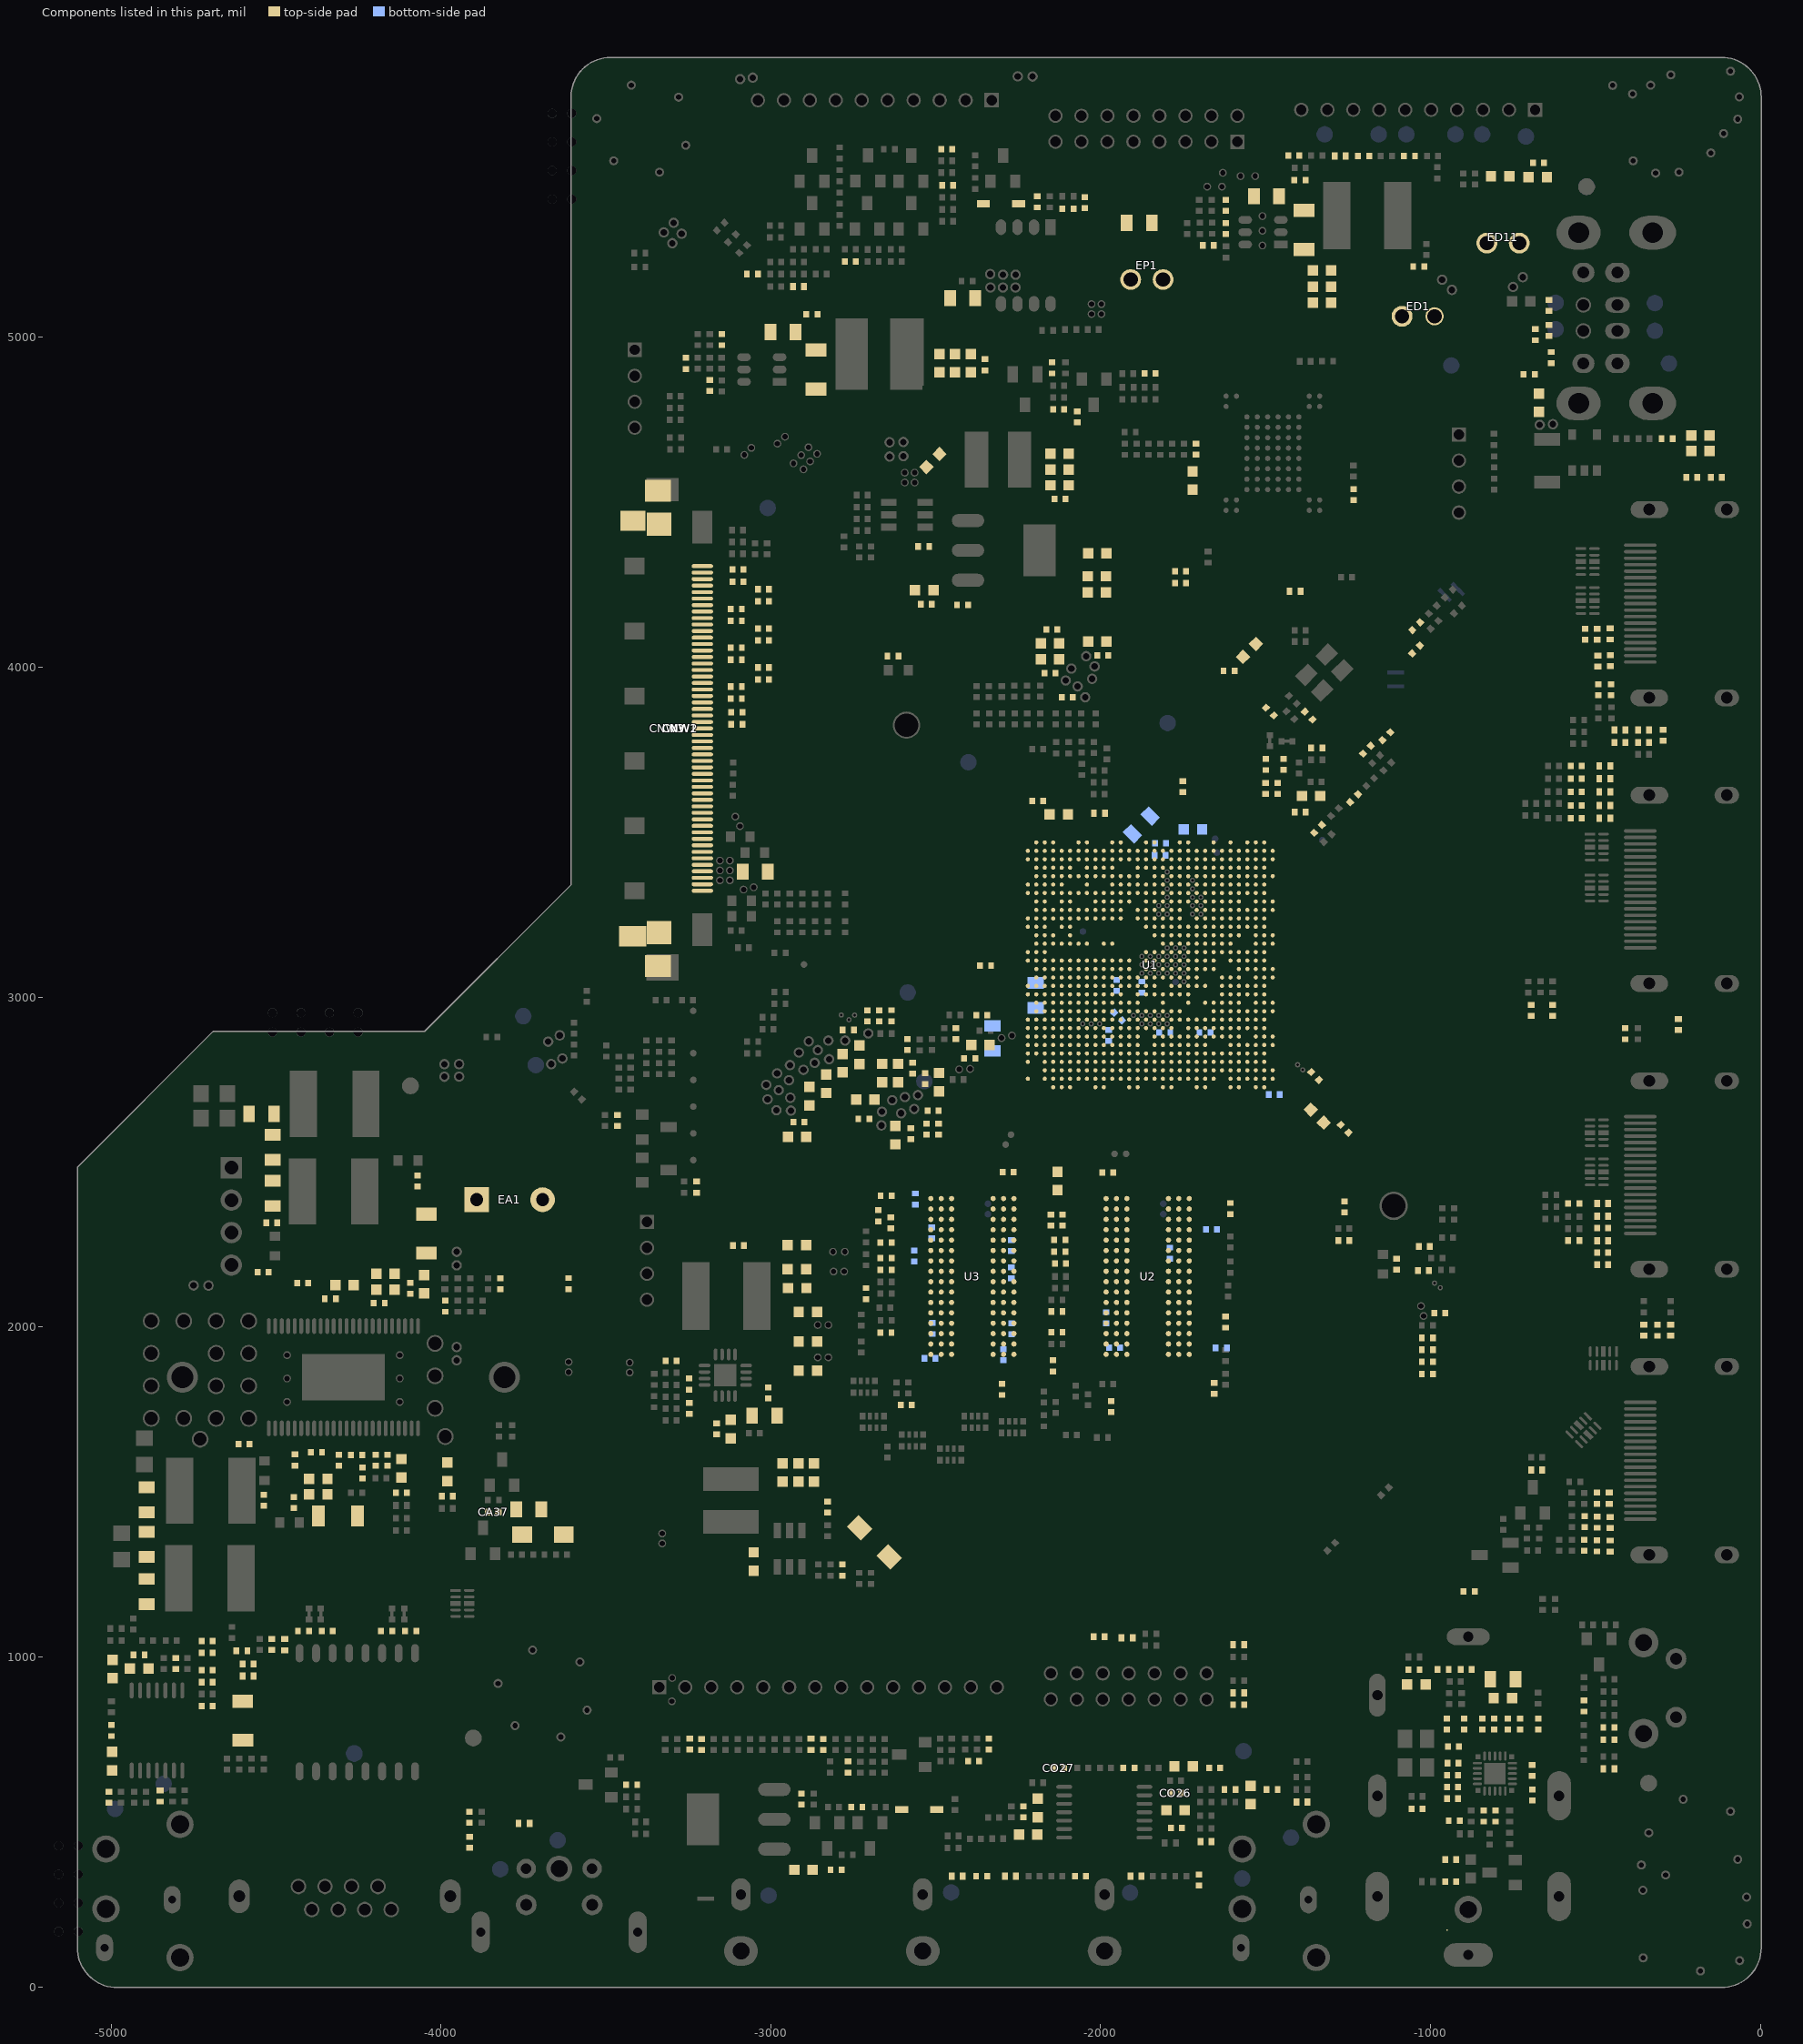
[diagram p0: the components of this part, seen from the top]
# Altium PCB MISC86290.PcbDoc (part 5 of 31)
Units mil, origin at the board's own origin, x right, y up, seen from the top; angles counter-clockwise.
Board outline 5104.71 x 5851.49 mil, 2 copper layers (TopLayer, BottomLayer), stack 61.855 mil thick; 1026 components, 667 nets, 4280 pads, 2294 vias.

## Footprints (in the part's own frame and the unit in brackets; to place one, negate y for a bottom-side part, rotate by r counter-clockwise, add the part's x,y. Pads: shape width x height; smd on the part's side, far side on the other; paste and mask are expansions set on the pad) (continued)
BGA96/0.8-1 [mm] "SKhynix；4GB DDR3 SDRAM　 9.4*13／NANYA　SDRAM B-Die　10*13兼容"
  round 0.4 smd: A1(-3.2,6) A2(-2.4,6) A3(-1.6,6) A7(1.6,6) A8(2.4,6) A9(3.2,6) B1(-3.2,5.2) B2(-2.4,5.2) B3(-1.6,5.2) B7(1.6,5.2) B8(2.4,5.2) B9(3.2,5.2) C1(-3.2,4.4) C2(-2.4,4.4) C3(-1.6,4.4) C7(1.6,4.4) C8(2.4,4.4) C9(3.2,4.4) D1(-3.2,3.6) D2(-2.4,3.6) D3(-1.6,3.6) D7(1.6,3.6) D8(2.4,3.6) D9(3.2,3.6) E1(-3.2,2.8) E2(-2.4,2.8) E3(-1.6,2.8) E7(1.6,2.8) E8(2.4,2.8) E9(3.2,2.8) F1(-3.2,2) F2(-2.4,2) F3(-1.6,2) F7(1.6,2) F8(2.4,2) F9(3.2,2) G1(-3.2,1.2) G2(-2.4,1.2) G3(-1.6,1.2) G7(1.6,1.2) G8(2.4,1.2) G9(3.2,1.2) H1(-3.2,0.4) H2(-2.4,0.4) H3(-1.6,0.4) H7(1.6,0.4) H8(2.4,0.4) H9(3.2,0.4) J1(-3.2,-0.4) J2(-2.4,-0.4) J3(-1.6,-0.4) J7(1.6,-0.4) J8(2.4,-0.4) J9(3.2,-0.4) K1(-3.2,-1.2) K2(-2.4,-1.2) K3(-1.6,-1.2) K7(1.6,-1.2) K8(2.4,-1.2) K9(3.2,-1.2) L1(-3.2,-2) L2(-2.4,-2) L3(-1.6,-2) L7(1.6,-2) L8(2.4,-2) L9(3.2,-2) M1(-3.2,-2.8) M2(-2.4,-2.8) M3(-1.6,-2.8) M7(1.6,-2.8) M8(2.4,-2.8) M9(3.2,-2.8) N1(-3.2,-3.6) N2(-2.4,-3.6) N3(-1.6,-3.6) N7(1.6,-3.6) N8(2.4,-3.6) N9(3.2,-3.6) P1(-3.2,-4.4) P2(-2.4,-4.4) P3(-1.6,-4.4) P7(1.6,-4.4) P8(2.4,-4.4) P9(3.2,-4.4) R1(-3.2,-5.2) R2(-2.4,-5.2) R3(-1.6,-5.2) R7(1.6,-5.2) R8(2.4,-5.2) R9(3.2,-5.2) T1(-3.2,-6) T2(-2.4,-6) T3(-1.6,-6) T7(1.6,-6) T8(2.4,-6) T9(3.2,-6)
  silkscreen extent -5.59,-6.7 5.05,7.49, body extent -5.05,-6.55 5.05,6.55, height 1.2
BGA758/0.65 [mm] "Mstar,MSDURN1801-Z1,0822_2018"
  round 0.32 smd mask+0.051: A2(-8.775,9.425) A3(-8.125,9.425) A5(-6.825,9.425) A6(-6.175,9.425) A9(-4.225,9.425) A10(-3.575,9.425) A13(-1.625,9.425) A14(-0.975,9.425) A17(0.975,9.425) A18(1.625,9.425) A21(3.575,9.425) A22(4.225,9.425) A25(6.175,9.425) A26(6.825,9.425) A27(7.475,9.425) AA2(-8.775,-3.575) AA3(-8.125,-3.575) AA4(-7.475,-3.575) AA5(-6.825,-3.575) AA6(-6.175,-3.575) AA7(-5.525,-3.575) AA8(-4.875,-3.575) AA9(-4.225,-3.575) AA10(-3.575,-3.575) AA12(-2.275,-3.575) AA13(-1.625,-3.575) AA14(-0.975,-3.575) AA15(-0.325,-3.575) AA16(0.325,-3.575) AA17(0.975,-3.575) AA19(2.275,-3.575) AA20(2.925,-3.575) AA21(3.575,-3.575) AA22(4.225,-3.575) AA23(4.875,-3.575) AA24(5.525,-3.575) AA25(6.175,-3.575) AA26(6.825,-3.575) AA27(7.475,-3.575) AA28(8.125,-3.575) AA29(8.775,-3.575) AA30(9.425,-3.575) AB1(-9.425,-4.225) AB2(-8.775,-4.225) AB3(-8.125,-4.225) AB4(-7.475,-4.225) AB5(-6.825,-4.225) AB6(-6.175,-4.225) AB7(-5.525,-4.225) AB8(-4.875,-4.225) AB9(-4.225,-4.225) AB10(-3.575,-4.225) AB12(-2.275,-4.225) AB13(-1.625,-4.225) AB14(-0.975,-4.225) AB15(-0.325,-4.225) AB16(0.325,-4.225) AB17(0.975,-4.225) AB19(2.275,-4.225) AB20(2.925,-4.225) AB21(3.575,-4.225) AB22(4.225,-4.225) AB23(4.875,-4.225) AB24(5.525,-4.225) AB25(6.175,-4.225) AB26(6.825,-4.225) AB27(7.475,-4.225) AB28(8.125,-4.225) AB29(8.775,-4.225) AC1(-9.425,-4.875) AC2(-8.775,-4.875) AC3(-8.125,-4.875) AC5(-6.825,-4.875) AC6(-6.175,-4.875) AC7(-5.525,-4.875) AC8(-4.875,-4.875) AC9(-4.225,-4.875) AC10(-3.575,-4.875) AC11(-2.925,-4.875) AC12(-2.275,-4.875) AC13(-1.625,-4.875) AC14(-0.975,-4.875) AC15(-0.325,-4.875) AC16(0.325,-4.875) AC18(1.625,-4.875) AC19(2.275,-4.875) AC20(2.925,-4.875) AC21(3.575,-4.875) AC22(4.225,-4.875) AC25(6.175,-4.875) AC26(6.825,-4.875) AC28(8.125,-4.875) AC29(8.775,-4.875) AD2(-8.775,-5.525) AD3(-8.125,-5.525) AD4(-7.475,-5.525) AD5(-6.825,-5.525) AD6(-6.175,-5.525) AD7(-5.525,-5.525) AD8(-4.875,-5.525) AD9(-4.225,-5.525) AD10(-3.575,-5.525) AD11(-2.925,-5.525) AD12(-2.275,-5.525) AD13(-1.625,-5.525) AD14(-0.975,-5.525) AD15(-0.325,-5.525) AD16(0.325,-5.525) AD17(0.975,-5.525) AD18(1.625,-5.525) AD19(2.275,-5.525) AD20(2.925,-5.525) AD21(3.575,-5.525) AD22(4.225,-5.525) AD23(4.875,-5.525) AD24(5.525,-5.525) AD25(6.175,-5.525) AD26(6.825,-5.525) AD27(7.475,-5.525) AD28(8.125,-5.525) AD29(8.775,-5.525) AD30(9.425,-5.525) AE2(-8.775,-6.175) AE3(-8.125,-6.175) AE4(-7.475,-6.175) AE5(-6.825,-6.175) AE6(-6.175,-6.175) AE7(-5.525,-6.175) AE8(-4.875,-6.175) AE9(-4.225,-6.175) AE10(-3.575,-6.175) AE11(-2.925,-6.175) AE12(-2.275,-6.175) AE13(-1.625,-6.175) AE14(-0.975,-6.175) AE15(-0.325,-6.175) AE16(0.325,-6.175) AE17(0.975,-6.175) AE18(1.625,-6.175) AE19(2.275,-6.175) AE20(2.925,-6.175) AE23(4.875,-6.175) AE26(6.825,-6.175) AE27(7.475,-6.175) AE28(8.125,-6.175) AE29(8.775,-6.175) AE30(9.425,-6.175) AF1(-9.425,-6.825) AF2(-8.775,-6.825) AF3(-8.125,-6.825) AF4(-7.475,-6.825) AF5(-6.825,-6.825) AF6(-6.175,-6.825) AF7(-5.525,-6.825) AF8(-4.875,-6.825) AF9(-4.225,-6.825) AF10(-3.575,-6.825) AF11(-2.925,-6.825) AF12(-2.275,-6.825) AF13(-1.625,-6.825) AF14(-0.975,-6.825) AF15(-0.325,-6.825) AF17(0.975,-6.825) AF18(1.625,-6.825) AF19(2.275,-6.825) AF20(2.925,-6.825) AF21(3.575,-6.825) AF22(4.225,-6.825) AF23(4.875,-6.825) AF24(5.525,-6.825) AF25(6.175,-6.825) AF26(6.825,-6.825) AF27(7.475,-6.825) AF28(8.125,-6.825) AF29(8.775,-6.825) AG2(-8.775,-7.475) AG3(-8.125,-7.475) AG4(-7.475,-7.475) AG5(-6.825,-7.475) AG6(-6.175,-7.475) AG7(-5.525,-7.475) AG8(-4.875,-7.475) AG9(-4.225,-7.475) AG10(-3.575,-7.475) AG11(-2.925,-7.475) AG12(-2.275,-7.475) AG13(-1.625,-7.475) AG14(-0.975,-7.475) AG15(-0.325,-7.475) AG16(0.325,-7.475) AG17(0.975,-7.475) AG20(2.925,-7.475) AG21(3.575,-7.475) AG22(4.225,-7.475) AG23(4.875,-7.475) AG25(6.175,-7.475) AG26(6.825,-7.475) AG27(7.475,-7.475) AG28(8.125,-7.475) AG29(8.775,-7.475) AH1(-9.425,-8.125) AH2(-8.775,-8.125) AH3(-8.125,-8.125) AH4(-7.475,-8.125) AH5(-6.825,-8.125) AH6(-6.175,-8.125) AH7(-5.525,-8.125) AH8(-4.875,-8.125) AH9(-4.225,-8.125) AH10(-3.575,-8.125) AH11(-2.925,-8.125) AH12(-2.275,-8.125) AH13(-1.625,-8.125) AH14(-0.975,-8.125) AH15(-0.325,-8.125) AH16(0.325,-8.125) AH17(0.975,-8.125) AH18(1.625,-8.125) AH19(2.275,-8.125) AH20(2.925,-8.125) AH21(3.575,-8.125) AH22(4.225,-8.125) AH23(4.875,-8.125) AH24(5.525,-8.125) AH25(6.175,-8.125) AH26(6.825,-8.125) AH27(7.475,-8.125) AH28(8.125,-8.125) AH29(8.775,-8.125) AH30(9.425,-8.125) AJ1(-9.425,-8.775) AJ2(-8.775,-8.775) AJ3(-8.125,-8.775) AJ4(-7.475,-8.775) AJ5(-6.825,-8.775) AJ6(-6.175,-8.775) AJ7(-5.525,-8.775) AJ8(-4.875,-8.775) AJ9(-4.225,-8.775) AJ10(-3.575,-8.775) AJ11(-2.925,-8.775) AJ12(-2.275,-8.775) AJ13(-1.625,-8.775) AJ14(-0.975,-8.775) AJ15(-0.325,-8.775) AJ16(0.325,-8.775) AJ17(0.975,-8.775) AJ18(1.625,-8.775) AJ19(2.275,-8.775) AJ20(2.925,-8.775) AJ21(3.575,-8.775) AJ22(4.225,-8.775) AJ23(4.875,-8.775) AJ24(5.525,-8.775) AJ25(6.175,-8.775) AJ26(6.825,-8.775) AJ27(7.475,-8.775) AJ28(8.125,-8.775) AJ29(8.775,-8.775) AJ30(9.425,-8.775) AK2(-8.775,-9.425) AK3(-8.125,-9.425) AK4(-7.475,-9.425) AK6(-6.175,-9.425) AK8(-4.875,-9.425) AK11(-2.925,-9.425) AK12(-2.275,-9.425) AK15(-0.325,-9.425) AK16(0.325,-9.425) AK19(2.275,-9.425) AK20(2.925,-9.425) AK23(4.875,-9.425) AK24(5.525,-9.425) AK27(7.475,-9.425) AK28(8.125,-9.425) AK29(8.775,-9.425) B1(-9.425,8.775) B2(-8.775,8.775) B3(-8.125,8.775) B4(-7.475,8.775) B5(-6.825,8.775) B6(-6.175,8.775) B8(-4.875,8.775) B9(-4.225,8.775) B10(-3.575,8.775) B11(-2.925,8.775) B12(-2.275,8.775) B13(-1.625,8.775) B14(-0.975,8.775) B15(-0.325,8.775) B16(0.325,8.775) B17(0.975,8.775) B18(1.625,8.775) B19(2.275,8.775) B20(2.925,8.775) B21(3.575,8.775) B22(4.225,8.775) B23(4.875,8.775) B24(5.525,8.775) B25(6.175,8.775) B26(6.825,8.775) B27(7.475,8.775) B28(8.125,8.775) B30(9.425,8.775) C1(-9.425,8.125) C2(-8.775,8.125) C3(-8.125,8.125) C4(-7.475,8.125) C5(-6.825,8.125) C6(-6.175,8.125) C7(-5.525,8.125) C8(-4.875,8.125) C9(-4.225,8.125) C10(-3.575,8.125) C11(-2.925,8.125) C12(-2.275,8.125) C13(-1.625,8.125) C14(-0.975,8.125) C15(-0.325,8.125) C16(0.325,8.125) C17(0.975,8.125) C18(1.625,8.125) C19(2.275,8.125) C20(2.925,8.125) C21(3.575,8.125) C22(4.225,8.125) C23(4.875,8.125) C24(5.525,8.125) C25(6.175,8.125) C26(6.825,8.125) C27(7.475,8.125) C28(8.125,8.125) D2(-8.775,7.475) D3(-8.125,7.475) D4(-7.475,7.475) D5(-6.825,7.475) D6(-6.175,7.475) D7(-5.525,7.475) D8(-4.875,7.475) D9(-4.225,7.475) D10(-3.575,7.475) D11(-2.925,7.475) D12(-2.275,7.475) D13(-1.625,7.475) D14(-0.975,7.475) D15(-0.325,7.475) D16(0.325,7.475) D17(0.975,7.475) D18(1.625,7.475) D19(2.275,7.475) D20(2.925,7.475) D21(3.575,7.475) D22(4.225,7.475) D23(4.875,7.475) D24(5.525,7.475) D25(6.175,7.475) D26(6.825,7.475) D27(7.475,7.475) D28(8.125,7.475) D30(9.425,7.475) E2(-8.775,6.825) E3(-8.125,6.825) E4(-7.475,6.825) E5(-6.825,6.825) E6(-6.175,6.825) E7(-5.525,6.825) E8(-4.875,6.825) E9(-4.225,6.825) E10(-3.575,6.825) E11(-2.925,6.825) E12(-2.275,6.825) E13(-1.625,6.825) E14(-0.975,6.825) E15(-0.325,6.825) E16(0.325,6.825) E17(0.975,6.825) E18(1.625,6.825) E19(2.275,6.825) E20(2.925,6.825) E21(3.575,6.825) E22(4.225,6.825) E23(4.875,6.825) E24(5.525,6.825) E25(6.175,6.825) E26(6.825,6.825) E27(7.475,6.825) E28(8.125,6.825) E29(8.775,6.825) E30(9.425,6.825) F1(-9.425,6.175) F2(-8.775,6.175) F3(-8.125,6.175) F4(-7.475,6.175) F5(-6.825,6.175) F6(-6.175,6.175) F9(-4.225,6.175) F10(-3.575,6.175) F11(-2.925,6.175) F12(-2.275,6.175) F13(-1.625,6.175) F14(-0.975,6.175) F15(-0.325,6.175) F17(0.975,6.175) F18(1.625,6.175) F19(2.275,6.175) F20(2.925,6.175) F21(3.575,6.175) F22(4.225,6.175) F23(4.875,6.175) F24(5.525,6.175) F25(6.175,6.175) F26(6.825,6.175) F27(7.475,6.175) F28(8.125,6.175) F29(8.775,6.175) F30(9.425,6.175) G1(-9.425,5.525) G2(-8.775,5.525) G3(-8.125,5.525) G5(-6.825,5.525) G6(-6.175,5.525) G7(-5.525,5.525) G8(-4.875,5.525) G9(-4.225,5.525) G10(-3.575,5.525) G11(-2.925,5.525) G12(-2.275,5.525) G13(-1.625,5.525) G14(-0.975,5.525) G15(-0.325,5.525) G17(0.975,5.525) G18(1.625,5.525) G19(2.275,5.525) G20(2.925,5.525) G21(3.575,5.525) G22(4.225,5.525) G23(4.875,5.525) G24(5.525,5.525) G25(6.175,5.525) G26(6.825,5.525) G27(7.475,5.525) G28(8.125,5.525) G29(8.775,5.525) G30(9.425,5.525) H2(-8.775,4.875) H3(-8.125,4.875) H4(-7.475,4.875) H5(-6.825,4.875) H6(-6.175,4.875) H7(-5.525,4.875) H8(-4.875,4.875) H9(-4.225,4.875) H10(-3.575,4.875) H11(-2.925,4.875) H13(-1.625,4.875) H14(-0.975,4.875) H15(-0.325,4.875) H16(0.325,4.875) H17(0.975,4.875) H18(1.625,4.875) H19(2.275,4.875) H20(2.925,4.875) H21(3.575,4.875) H22(4.225,4.875) H23(4.875,4.875) H24(5.525,4.875) H25(6.175,4.875) H26(6.825,4.875) H27(7.475,4.875) H28(8.125,4.875) H29(8.775,4.875) H30(9.425,4.875) J2(-8.775,4.225) J3(-8.125,4.225) J4(-7.475,4.225) J5(-6.825,4.225) J6(-6.175,4.225) J7(-5.525,4.225) J8(-4.875,4.225) J9(-4.225,4.225) J10(-3.575,4.225) J11(-2.925,4.225) J12(-2.275,4.225) J13(-1.625,4.225) J14(-0.975,4.225) J15(-0.325,4.225) J16(0.325,4.225) J17(0.975,4.225) J18(1.625,4.225) J19(2.275,4.225) J20(2.925,4.225) J21(3.575,4.225) J22(4.225,4.225) J23(4.875,4.225) J24(5.525,4.225) J25(6.175,4.225) J26(6.825,4.225) J27(7.475,4.225) J28(8.125,4.225) J29(8.775,4.225) J30(9.425,4.225) K1(-9.425,3.575) K2(-8.775,3.575) K3(-8.125,3.575) K4(-7.475,3.575) K5(-6.825,3.575) K6(-6.175,3.575) K7(-5.525,3.575) K8(-4.875,3.575) K12(-2.275,3.575) K13(-1.625,3.575) K14(-0.975,3.575) K15(-0.325,3.575) K16(0.325,3.575) K17(0.975,3.575) K18(1.625,3.575) K19(2.275,3.575) K20(2.925,3.575) K21(3.575,3.575) K22(4.225,3.575) K23(4.875,3.575) K24(5.525,3.575) K25(6.175,3.575) K26(6.825,3.575) K27(7.475,3.575) K28(8.125,3.575) K29(8.775,3.575) L1(-9.425,2.925) L2(-8.775,2.925) L3(-8.125,2.925) L5(-6.825,2.925) L6(-6.175,2.925) L7(-5.525,2.925) L8(-4.875,2.925) L9(-4.225,2.925) L11(-2.925,2.925) L14(-0.975,2.925) L17(0.975,2.925) L18(1.625,2.925) L19(2.275,2.925) L20(2.925,2.925) L21(3.575,2.925) L22(4.225,2.925) L23(4.875,2.925) L24(5.525,2.925) L25(6.175,2.925) L26(6.825,2.925) L27(7.475,2.925) L28(8.125,2.925) L29(8.775,2.925) M2(-8.775,2.275) M3(-8.125,2.275) M4(-7.475,2.275) M5(-6.825,2.275) M6(-6.175,2.275) M7(-5.525,2.275) M11(-2.925,2.275) M12(-2.275,2.275) M13(-1.625,2.275) M14(-0.975,2.275) M15(-0.325,2.275) M16(0.325,2.275) M17(0.975,2.275) M19(2.275,2.275) M20(2.925,2.275) M21(3.575,2.275) M22(4.225,2.275) M23(4.875,2.275) M24(5.525,2.275) M25(6.175,2.275) M26(6.825,2.275) M27(7.475,2.275) M28(8.125,2.275) M29(8.775,2.275) M30(9.425,2.275) N2(-8.775,1.625) N3(-8.125,1.625) N4(-7.475,1.625) N5(-6.825,1.625) N6(-6.175,1.625) N7(-5.525,1.625) N9(-4.225,1.625) N10(-3.575,1.625) N11(-2.925,1.625) N12(-2.275,1.625) N13(-1.625,1.625) N15(-0.325,1.625) N16(0.325,1.625) N17(0.975,1.625) N18(1.625,1.625) N19(2.275,1.625) N20(2.925,1.625) N21(3.575,1.625) N22(4.225,1.625) N23(4.875,1.625) N24(5.525,1.625) N25(6.175,1.625) N26(6.825,1.625) N27(7.475,1.625) N28(8.125,1.625) N29(8.775,1.625) N30(9.425,1.625) P1(-9.425,0.975) P2(-8.775,0.975) P3(-8.125,0.975) P5(-6.825,0.975) P6(-6.175,0.975) P7(-5.525,0.975) P10(-3.575,0.975) P11(-2.925,0.975) P12(-2.275,0.975) P13(-1.625,0.975) P14(-0.975,0.975) P15(-0.325,0.975) P16(0.325,0.975) P17(0.975,0.975) P18(1.625,0.975) P19(2.275,0.975) P20(2.925,0.975) P21(3.575,0.975) P22(4.225,0.975) P23(4.875,0.975) P24(5.525,0.975) P25(6.175,0.975) P26(6.825,0.975) P27(7.475,0.975) P28(8.125,0.975) P29(8.775,0.975) R1(-9.425,0.325) R2(-8.775,0.325) R3(-8.125,0.325) R4(-7.475,0.325) R5(-6.825,0.325) R8(-4.875,0.325) R9(-4.225,0.325) R10(-3.575,0.325) R11(-2.925,0.325) R12(-2.275,0.325) R13(-1.625,0.325) R14(-0.975,0.325) R15(-0.325,0.325) R16(0.325,0.325) R18(1.625,0.325) R19(2.275,0.325) R20(2.925,0.325) R21(3.575,0.325) R22(4.225,0.325) R23(4.875,0.325) R24(5.525,0.325) R25(6.175,0.325) R26(6.825,0.325) R27(7.475,0.325) R28(8.125,0.325) R29(8.775,0.325) T2(-8.775,-0.325) T3(-8.125,-0.325) T4(-7.475,-0.325) T5(-6.825,-0.325) T6(-6.175,-0.325) T8(-4.875,-0.325) T9(-4.225,-0.325) T10(-3.575,-0.325) T11(-2.925,-0.325) T12(-2.275,-0.325) T13(-1.625,-0.325) T14(-0.975,-0.325) T15(-0.325,-0.325) T16(0.325,-0.325) T18(1.625,-0.325) T19(2.275,-0.325) T20(2.925,-0.325) T21(3.575,-0.325) T22(4.225,-0.325) T23(4.875,-0.325) T24(5.525,-0.325) T25(6.175,-0.325) T26(6.825,-0.325) T27(7.475,-0.325) T28(8.125,-0.325) T29(8.775,-0.325) T30(9.425,-0.325) U2(-8.775,-0.975) U3(-8.125,-0.975) U4(-7.475,-0.975) U5(-6.825,-0.975) U6(-6.175,-0.975) U7(-5.525,-0.975) U8(-4.875,-0.975) U9(-4.225,-0.975) U10(-3.575,-0.975) U11(-2.925,-0.975) U12(-2.275,-0.975) U13(-1.625,-0.975) U14(-0.975,-0.975) U15(-0.325,-0.975) U16(0.325,-0.975) U28(8.125,-0.975) U29(8.775,-0.975) U30(9.425,-0.975) V1(-9.425,-1.625) V2(-8.775,-1.625) V3(-8.125,-1.625) V6(-6.175,-1.625) V7(-5.525,-1.625) V8(-4.875,-1.625) V9(-4.225,-1.625) V10(-3.575,-1.625) V11(-2.925,-1.625) V12(-2.275,-1.625) V13(-1.625,-1.625) V14(-0.975,-1.625) V20(2.925,-1.625) V21(3.575,-1.625) V23(4.875,-1.625) V24(5.525,-1.625) V25(6.175,-1.625) V26(6.825,-1.625) V27(7.475,-1.625) V28(8.125,-1.625) V29(8.775,-1.625) W1(-9.425,-2.275) W2(-8.775,-2.275) W3(-8.125,-2.275) W5(-6.825,-2.275) W6(-6.175,-2.275) W7(-5.525,-2.275) W8(-4.875,-2.275) W9(-4.225,-2.275) W10(-3.575,-2.275) W11(-2.925,-2.275) W12(-2.275,-2.275) W13(-1.625,-2.275) W14(-0.975,-2.275) W15(-0.325,-2.275) W25(6.175,-2.275) W27(7.475,-2.275) W28(8.125,-2.275) W29(8.775,-2.275) Y2(-8.775,-2.925) Y3(-8.125,-2.925) Y4(-7.475,-2.925) Y5(-6.825,-2.925) Y6(-6.175,-2.925) Y7(-5.525,-2.925) Y8(-4.875,-2.925) Y9(-4.225,-2.925) Y10(-3.575,-2.925) Y11(-2.925,-2.925) Y12(-2.275,-2.925) Y13(-1.625,-2.925) Y14(-0.975,-2.925) Y15(-0.325,-2.925) Y16(0.325,-2.925) Y25(6.175,-2.925) Y26(6.825,-2.925) Y28(8.125,-2.925) Y29(8.775,-2.925) Y30(9.425,-2.925)
  silkscreen extent -11.02,-10.15 10.15,10.85, body extent -10.15,-10.15 10.15,10.15, height 1.55
C0402#1 [mm] "片式电容"
  rect 0.45x0.5 smd mask+0.076: 1(-0.425,0) 2(0.425,0)
  silkscreen extent -0.88,-0.4 0.88,0.4, body extent -0.5,-0.25 0.5,0.25, height 0.5
C0402#2 [mm] "片式电容  2018.10.7 替换为兼容0201封装"
  rrect50% 0.45x0.5 smd mask+0.051: 1(-0.425,0) 2(0.425,0)
  rect 0.3x0.3 smd mask+0.051: 1(-0.25,0) 2(0.25,0)
  rect 0.6x0.6 on Top Solder: 2(0,0)
  TopLayer pour cut-out: -0.318,0.302 -0.318,-0.303 0.306,-0.303 0.306,0.302
  silkscreen extent -0.88,-0.4 0.88,0.4, body extent -0.5,-0.25 0.5,0.25, height 0.5
C0402#3 [mm] "片式电容"
  rect 0.45x0.5 smd mask+0.076: 1(-0.425,0) 1(-0.425,0) 2(0.425,0) 2(0.425,0)
  silkscreen extent -0.88,-0.4 0.88,0.4, body extent -0.5,-0.25 0.5,0.25, height 0.5
C0603 [mm] "片式电容"
  rect 0.8x0.8 smd mask+0.076: 1(-0.706,0) 2(0.706,0)
  silkscreen extent -1.39,-0.55 1.39,0.55, body extent -0.8,-0.4 0.8,0.4, height 0.8
C0805 [mm] "片式电容"
  rect 0.9x1.25 smd mask+0.076: 1(-0.966,0) 2(0.966,0)
  silkscreen extent -1.73,-0.78 1.73,0.78, body extent -1,-0.63 1,0.63, height 1.25
C1206 [mm] "片式电容"
  rect 1x1.6 smd mask+0.076: 1(-1.5,-0.001) 2(1.5,0.001)
  silkscreen extent -2.39,-0.95 2.39,0.95, body extent -1.6,-0.8 1.6,0.8, height 1.3
CQC [mil]
DIODE-S0402 [mm] "DVD上使用的ESD"
  rect 0.45x0.55 smd mask+0.051: A(-0.425,0) K(0.425,0)
  silkscreen extent -0.8,-0.43 0.91,0.43, body extent -0.5,-0.25 0.5,0.25, height 0.5
DIODE-S0805 [mil] "1N4148"
  rect 60x50 smd: A(-62.99,0) K(62.99,0)
  silkscreen extent -114,-39 114,39, body extent -69,-24 69,24, height 49
DIODE-S-12 [mm] "Formosa MS ;BAV19WS THRU BAV21WS/PMEG2010BEA(高度为1.1mm)"
  rect 1x0.55 smd: A(1.35,0) K(-1.35,0)
  silkscreen extent -0.9,-0.67 0.9,0.67, body extent -1.35,-0.63 1.35,0.63, height 1
"DOLBY PLUS-SILK" [mil]
  silkscreen extent -16,-177 1441,197
EC(6.3*11)-V-2.5#1 [mm] "机插2.5间距"
  round 0.5 on Keep-Out: 0(0.562,1.527)
  round 1.6 hole 1.1: 1(-1.25,0)
  round 1.4 / inner round 1.6 / far side round 1.6 hole 1.1: 2(1.25,0)
  round 1.8 on Top Overlay: 5(1.25,0) 6(-1.25,0)
  BottomLayer lines w0.6: -1.665,-0.275 -1.691,-0.225 -2.664,1.685 ; -1.25,0 -2.664,1.685 ; -0.907,0.361 -0.952,0.395 ; 0.907,-0.361 2.664,-1.685 ; 1.25,0 2.664,-1.685 ; 1.665,0.275 2.664,-1.685 ; -2.664,1.685 -0.952,0.395 ; -0.952,0.395 -0.952,0.395 ; -0.952,0.395 -0.952,0.395
  silkscreen extent -3.17,-3.17 3.51,3.17, body extent -3,-3 2.98,2.99, height 12.5
EC(6.3*11)-V-2.5#2 [mm] "机插2.5间距"
  round 0.5 on Keep-Out: 0(0,0.889)
  round 1.6 hole 1.1: 1(-1.25,0) 2(1.25,0)
  round 1.8 on Top Overlay: 5(1.25,0) 6(-1.25,0)
  BottomLayer lines w0.6: -1.665,-0.275 -1.691,-0.225 -2.664,1.685 ; -1.25,0 -2.664,1.685 ; -0.907,0.361 -0.952,0.395 -2.664,1.685 ; 0.907,-0.361 2.664,-1.685 ; 1.25,0 2.664,-1.685 ; 1.665,0.275 2.664,-1.685
  silkscreen extent -3.17,-3.17 3.51,3.17, body extent -3,-3 2.98,2.99, height 12.5
EC(6.3*11)-V-2.5#3 [mm] "机插2.5间距"
  round 0.5 on Keep-Out: 0(-0.508,2.162)
  round 1.6 hole 1.1: 1(-1.25,0) 2(1.25,0)
  round 1.8 on Top Overlay: 5(1.25,0) 6(-1.25,0)
  BottomLayer lines w0.6: -1.665,-0.275 -1.691,-0.225 -2.664,1.685 ; -1.25,0 -2.664,1.685 ; -0.907,0.361 -0.952,0.395 ; 0.907,-0.361 2.664,-1.685 ; 1.25,0 2.664,-1.685 ; 1.665,0.275 2.664,-1.685 ; -2.664,1.685 -0.952,0.395 ; -0.952,0.395 -0.952,0.395 ; -0.952,0.395 -0.952,0.395
  silkscreen extent -3.17,-3.17 3.51,3.17, body extent -3,-3 2.98,2.99, height 12.5
EC(10*13)-V-5.0-1 [mm] "470uF-35V-±20%-10×13-105℃-黑底白字-编带F=5.0-XF;14.05.21"
  rect 2.1x2.1 on Top Overlay: 0(-2.54,0)
  round 0.5 on Keep-Out: 0(0,0)
  round 2.1 on Top Overlay: 0(2.54,0)
  rect 1.9x1.9 hole 1: 1(-2.54,0)
  round 1.9 hole 1: 2(2.54,0)
  BottomLayer lines w0.6: -3.063,-0.387 -3.108,-0.302 -4.096,1.556 ; -2.54,0 -4.096,1.556 ; -2.153,0.523 -2.238,0.568 -4.096,1.556 ; 2.153,-0.523 4.096,-1.556 ; 2.54,0 4.096,-1.556 ; 3.063,0.387 4.096,-1.556
  silkscreen extent -5.25,-5.25 5.4,5.25, body extent -4.98,-4.99 5.01,4.99, height 14.51
ESD [mm]
  round 0.1 smd paste-0.1 mask-0.1: 1(0.835,0.002) 2(-0.824,0.014)
  TopLayer pour cut-out: -1.172,0.278 1.172,0.278 1.172,-0.28 -1.172,-0.28
  TopLayer lines w0.025: -1.171,0 -1.151,0 ; 1.172,-0.858 0.938,-0.858 ; 1.172,-0.858 1.172,0.838 ; 1.172,-0.858 0.938,-0.858 ; 1.172,-0.858 1.172,0.838 ; 0.938,-0.858 0.08,0 ; 0.938,-0.858 0.08,0 ; 1.172,0.838 0.918,0.838 ; 1.172,0.838 0.918,0.838 ; 0.111,0 0.947,-0.836 1.151,-0.836 1.151,0.817 1.159,0.825 0.936,0.825 0.111,0 ; 0.111,0 0.08,0 ; 0.111,0 0.111,0 ; 0.918,0.838 0.08,0 ; 0.918,0.838 0.08,0 ; 0.08,0 1.171,0 0.08,0 ; -0.08,0 -0.772,0.692 -0.938,0.858 -1.172,0.858 -1.172,0.024 -1.172,-0.006 -1.172,-0.02 -1.172,-0.553 -1.172,-0.838 -0.947,-0.838 -0.918,-0.838 -0.748,-0.668 -0.734,-0.654 -0.08,0 ; -0.08,0 -0.111,0 ; -0.08,0 -0.111,0 ; -0.111,0 -0.787,0.676 -0.947,0.836 -1.151,0.836 -1.151,0.024 -1.151,0 ; -0.111,0 -0.744,-0.633 -0.764,-0.652 -0.936,-0.825 -0.956,-0.825 -1.159,-0.825 -1.151,-0.817 -1.151,-0.576 -1.151,-0.02 -1.151,-0.006 -1.151,0 ; -0.111,0 -0.35,0 -0.375,0 -0.621,0 -0.824,0 -0.964,0 -1.096,0 -1.151,0 ; -0.111,0 -0.111,0
  TopLayer lines w0.127: 0.964,-0.622 0.964,-0.645 1.101,-0.781 0.992,-0.781 1.063,-0.71 1.113,-0.71 1.096,-0.693 1.096,0.766 1.08,0.782 0.955,0.782 0.627,0.454 0.79,0.454 ; 1.116,-0.005 0.16,-0.005 ; 0.367,-0.048 0.828,-0.509 0.828,-0.622 0.304,-0.098 0.277,-0.098 ; 0.505,0.313 0.498,0.313 0.301,0.116 ; -0.16,0.005 -0.621,0.005 -0.824,0.005 -0.964,0.005 -1.096,0.005 ; -0.301,-0.116 -0.498,-0.313 -0.505,-0.313 ; -0.79,-0.454 -0.627,-0.454 -0.765,-0.591 -0.795,-0.621 -0.947,-0.774 -0.955,-0.781 -0.955,-0.782 -0.986,-0.782 -1.08,-0.782 -1.096,-0.766 -1.096,-0.641 -1.096,-0.132 -1.096,-0.02 -1.096,-0.006 -1.096,0 -1.096,0.005 ; -0.277,0.098 -0.304,0.098 -0.828,0.622 -0.828,0.509 -0.367,0.048 ; -1.116,0.005 -1.096,0.005 ; -0.964,0.622 -0.964,0.645 -1.007,0.688 -1.014,0.695 -1.046,0.727 ; -1.096,0.005 -1.096,0.024 -1.096,0.693 -1.113,0.71 -1.063,0.71 -1.046,0.727 ; -1.046,0.727 -1.101,0.781 -0.992,0.781 -1.046,0.727
  TopLayer lines w0.381: 0.964,-0.622 0.964,0.615 ; 0.621,-0.277 0.621,0.29 ; 0.375,0 0.35,0 ; -0.621,-0.29 -0.621,-0.02 -0.621,-0.006 -0.621,0 -0.621,0.005 -0.621,0.014 -0.621,0.024 -0.621,0.277 ; -0.964,-0.615 -0.964,-0.281 -0.964,-0.02 -0.964,-0.006 -0.964,0 -0.964,0.005 -0.964,0.014 ; -0.35,0 -0.375,0 ; -0.964,0.622 -0.964,0.024 -0.964,0.014 ; -0.964,0.014 -0.964,0.014
FFC51-H/0.5S-1 [mm] "深圳得康   FPC0.5-51P卧贴后掀盖90°,翻盖后高度6.4mm/新富尔，0.5G-nPBX;170106优化焊盘"
  oval 0.3x1.65 smd: 1(-12.5,1.56) 2(-12,1.56) 3(-11.5,1.56) 4(-11,1.56) 5(-10.5,1.56) 6(-10,1.56) 7(-9.5,1.56) 8(-9,1.56) 9(-8.5,1.56) 10(-8,1.56) 11(-7.5,1.56) 12(-7,1.56) 13(-6.5,1.56) 14(-6,1.56) 15(-5.5,1.56) 16(-5,1.56) 17(-4.5,1.56) 18(-4,1.56) 19(-3.5,1.56) 20(-3,1.56) 21(-2.5,1.56) 22(-2,1.56) 23(-1.5,1.56) 24(-1,1.56) 25(-0.5,1.56) 26(0,1.56) 27(0.5,1.56) 28(1,1.56) 29(1.5,1.56) 30(2,1.56) 31(2.5,1.56) 32(3,1.56) 33(3.5,1.56) 34(4,1.56) 35(4.5,1.56) 36(5,1.56) 37(5.5,1.56) 38(6,1.56) 39(6.5,1.56) 40(7,1.56) 41(7.5,1.56) 42(8,1.56) 43(8.5,1.56) 44(9,1.56) 45(9.5,1.56) 46(10,1.56) 47(10.5,1.56) 48(11,1.56) 49(11.5,1.56) 50(12,1.56) 51(12.5,1.56)
  rect 1.8x1.9 smd: 52(15.72,-1.76) 53(-15.72,-1.76)
  silkscreen extent -16,-5.27 16,3.41
FFC51H/0.5S-10 [mm] "DEREN,78-050251019,翻盖高度5.65mm;16.12.09(替换FFC51H/0.5S-7）;170405更新丝印突出长度"
  oval 0.26x1.55 smd mask+0.076: 1(-12.5,1.716) 2(-12,1.716) 3(-11.5,1.717) 4(-11,1.717) 5(-10.5,1.716) 6(-10,1.716) 7(-9.5,1.716) 8(-9,1.716) 9(-8.5,1.716) 10(-8,1.717) 11(-7.5,1.716) 12(-7,1.716) 13(-6.5,1.716) 14(-6,1.716) 15(-5.5,1.716) 16(-5,1.716) 17(-4.5,1.716) 18(-4,1.716) 19(-3.5,1.716) 20(-3,1.716) 21(-2.5,1.716) 22(-2,1.716) 23(-1.5,1.716) 24(-1,1.717) 25(-0.5,1.716) 26(0,1.716) 27(0.5,1.716) 28(1,1.716) 29(1.5,1.716) 30(2,1.717) 31(2.5,1.717) 32(3,1.717) 33(3.5,1.716) 34(4,1.716) 35(4.5,1.716) 36(5,1.716) 37(5.5,1.716) 38(6,1.716) 39(6.5,1.716) 40(7,1.716) 41(7.5,1.716) 42(8,1.716) 43(8.5,1.716) 44(9,1.716) 45(9.5,1.716) 46(10,1.716) 47(10.5,1.716) 48(11,1.716) 49(11.5,1.716) 50(12,1.717) 51(12.5,1.716)
  rect 1.66x2 smd mask+0.076: 52(-18.3,-1.716) 53(18.3,-1.716)
  silkscreen extent -17.75,-5.72 17.74,3.66
FFC51H/0.5S-12 [mm] "昶通;F05035FA51M1WL,翻开高度5.3mm);17.11.07"
  rect 0.25x1.2 smd: 1(-12.5,2.825)
  oval 0.25x1.2 smd: 2(-12,2.825) 3(-11.5,2.825) 4(-11,2.825) 5(-10.5,2.825) 6(-10,2.825) 7(-9.5,2.825) 8(-9,2.825) 9(-8.5,2.825) 10(-8,2.825) 11(-7.5,2.825) 12(-7,2.825) 13(-6.5,2.825) 14(-6,2.825) 15(-5.5,2.825) 16(-5,2.825) 17(-4.5,2.825) 18(-4,2.825) 19(-3.5,2.825) 20(-3,2.825) 21(-2.5,2.825) 22(-2,2.825) 23(-1.5,2.825) 24(-1,2.825) 25(-0.5,2.825) 26(0,2.825) 27(0.5,2.825) 28(1,2.825) 29(1.5,2.825) 30(2,2.825) 31(2.5,2.825) 32(3,2.825) 33(3.5,2.825) 34(4,2.825) 35(4.5,2.825) 36(5,2.825) 37(5.5,2.825) 38(6,2.825) 39(6.5,2.825) 40(7,2.825) 41(7.5,2.825) 42(8,2.825) 43(8.5,2.825) 44(9,2.825) 45(9.5,2.825) 46(10,2.825) 47(10.5,2.825) 48(11,2.825) 49(11.5,2.825) 50(12,2.825) 51(12.5,2.825)
  rect 1.6x2.1 smd: 52(16,-2.525)
  rect 1.524x1.93 smd: 53(-16,-2.525)
  silkscreen extent -16.35,-4.66 16.35,4.37